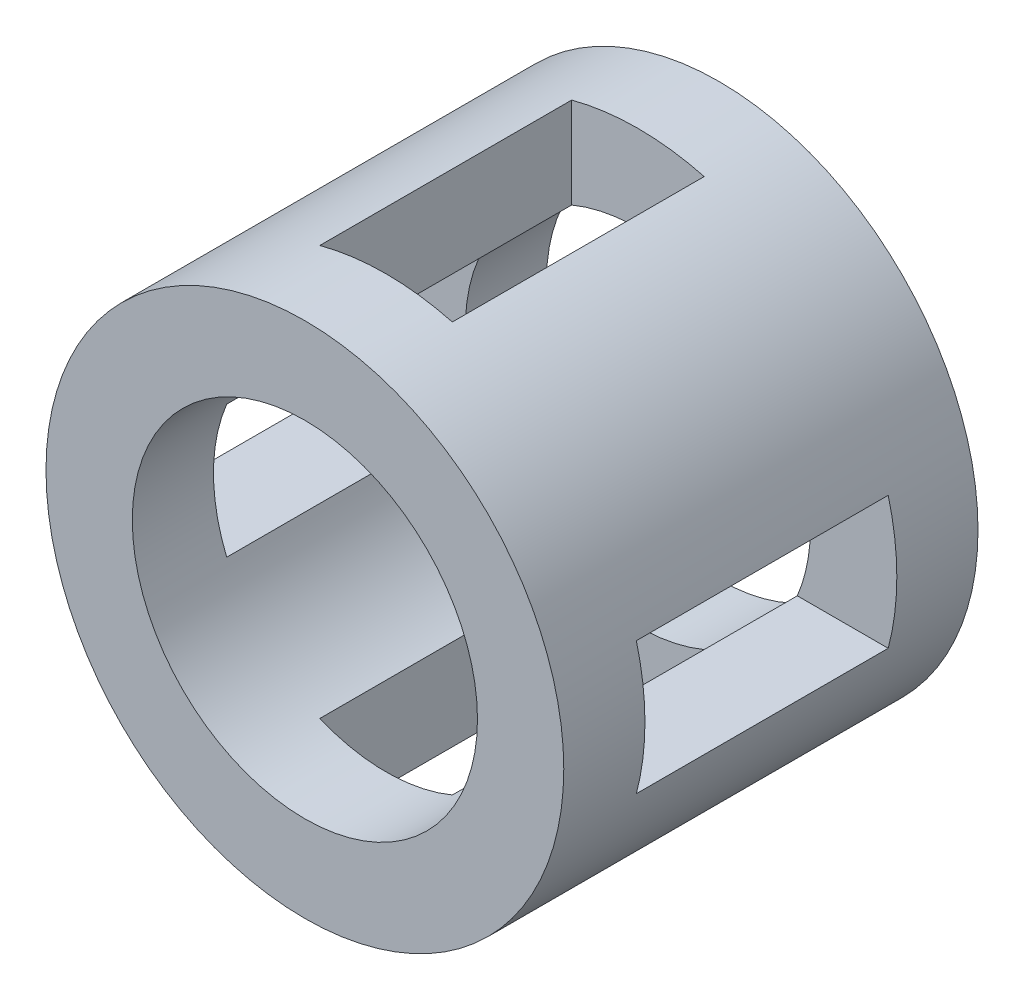
SolidWorks part; units mm, degrees
ref_plane "Front Plane" through (0, 0, 0) normal (0, 0, 1) x (1, 0, 0)
ref_plane "Top Plane" through (0, 0, 0) normal (0, 1, 0) x (1, 0, 0)
ref_plane "Right Plane" through (0, 0, 0) normal (1, 0, 0) x (0, 0, -1)
sketch "Sketch1" plane through (0, 0, 0) normal (0, 0, 1) x (1, 0, 0)
  circle A0 centre (0, 0) radius 75
  circle A1 centre (0, 0) radius 50
  dimension "D1" = 150
  dimension "D2" = 100
extrude "Boss-Extrude1" add sketch "Sketch1" along normal blind 120
sketch "Sketch2" plane through (0, 0, 0) normal (0, 1, 0) x (1, 0, 0)
  line L1 (-19.1956, -23.5157) -> (19.1956, -23.5157)
  line L2 (-19.1956, -23.5157) -> (-19.1956, -96.4843)
  line L3 (-19.1956, -96.4843) -> (19.1956, -96.4843)
  line L4 (19.1956, -23.5157) -> (19.1956, -96.4843)
  line L5 (-19.1956, -23.5157) -> (19.1956, -96.4843) construction
  line L6 (-19.1956, -96.4843) -> (19.1956, -23.5157) construction
  point P0 (0, -60)
extrude "Cut-Extrude1" cut sketch "Sketch2" against normal through all
pattern_circular "CirPattern1" count 4 over 360 about axis through (0, 0, 0) along (0, 0, 1) of "Cut-Extrude1"
